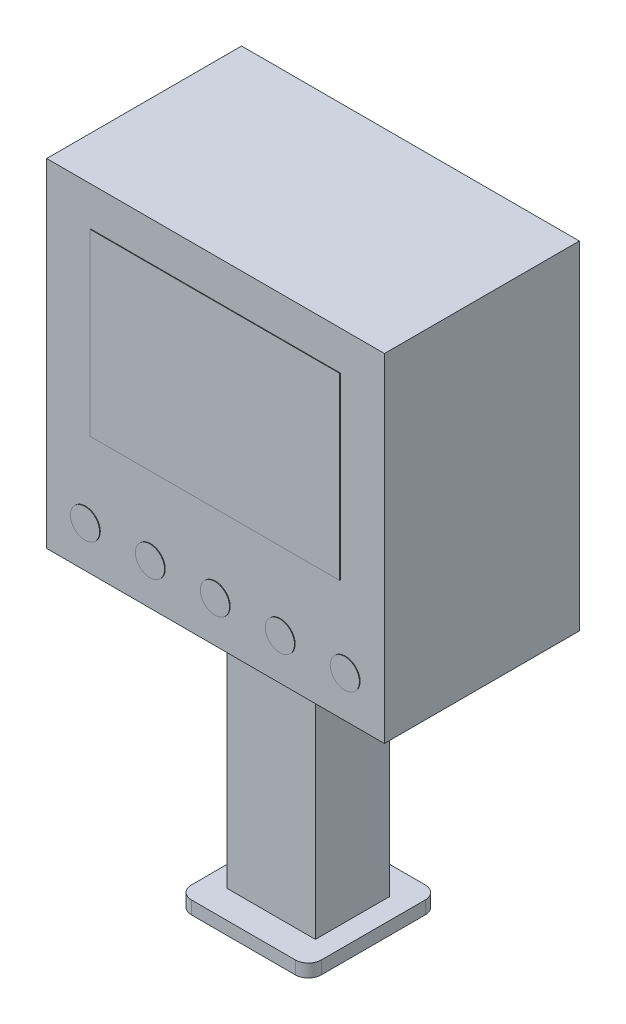
from build123d import *

# Parameters (mm, degrees)
SKETCH1_W           = 260
SKETCH1_H           = 260
BOSS_EXTRUDE1_DEPTH = 150
SKETCH2_R           = 11.25
SKETCH2_W           = 192
SKETCH2_H           = 138
BOSS_EXTRUDE2_DEPTH = 0.5
SKETCH3_W           = 68.073396254
SKETCH3_H           = 57.221115693
BOSS_EXTRUDE3_DEPTH = 200
SKETCH4_W           = 100
SKETCH4_H           = 100
BOSS_EXTRUDE4_DEPTH = 10
FILLET1_R           = 10


with BuildPart() as part:
    # Sketch1 → Boss-Extrude1 (new body)
    with BuildSketch(Plane.XY):
        Rectangle(SKETCH1_W, SKETCH1_H)
    extrude(amount=BOSS_EXTRUDE1_DEPTH)

    # Sketch2 → Boss-Extrude2 (add)
    with BuildSketch(Plane.XY.offset(150)):
        with Locations((-100, -98)):
            Circle(SKETCH2_R)
        with Locations((-50, -98)):
            Circle(SKETCH2_R)
        with Locations(Location((50, -98, 0), (0, 0, 180))):
            Circle(SKETCH2_R)
        with Locations(Location((100, -98, 0), (0, 0, 180))):
            Circle(SKETCH2_R)
        with Locations(Location((0, -98, 0), (0, 0, 180))):
            Circle(SKETCH2_R)
        with Locations((0, 31)):
            Rectangle(SKETCH2_W, SKETCH2_H)
    extrude(amount=BOSS_EXTRUDE2_DEPTH)

    # Sketch3 → Boss-Extrude3 (add)
    with BuildSketch(Plane.XZ.offset(130)):
        with Locations((0, 78.579676991)):
            Rectangle(SKETCH3_W, SKETCH3_H)
    extrude(amount=BOSS_EXTRUDE3_DEPTH)

    # Sketch4 → Boss-Extrude4 (add)
    with BuildSketch(Plane.XZ.offset(330)):
        with Locations((0, 78.579676991)):
            Rectangle(SKETCH4_W, SKETCH4_H)
    extrude(amount=BOSS_EXTRUDE4_DEPTH)

    # Fillet1
    fillet1_edges = [part.edges().sort_by_distance(p)[0] for p in [
        (50, -335, 28.579676991),
        (50, -335, 128.579676991),
        (-50, -335, 128.579676991),
        (-50, -335, 28.579676991),
    ]]
    fillet(fillet1_edges, radius=FILLET1_R)


solid = part.part
